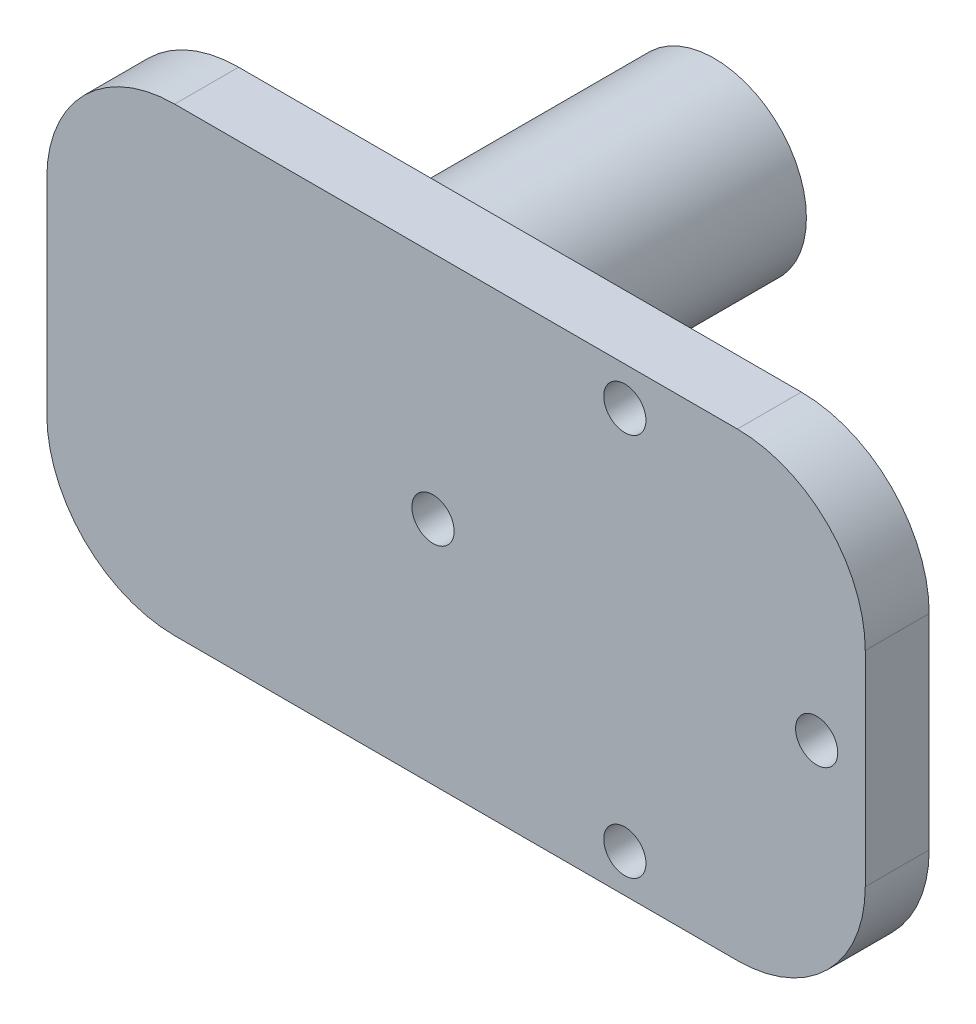
from build123d import *

# Parameters (mm, degrees)
SKETCH_1_R               = 7.2
SKETCH_1_R_2             = 4.2
EXTRUDE_1_DEPTH          = 7.5
EXTRUDE_START            = 20
SKETCH_2_R               = 7.2
EXTRUDE_2_DEPTH          = 20
SKETCH_3_R               = 17.2
SKETCH_3_R_2             = 7.2
EXTRUDE_3_DEPTH          = 3
SKETCH_4_R               = 1.65
CUT_EXTRUDE_1_DEPTH      = 3
PATTERN_CIRCULAR_1_COUNT = 4
SKETCH_5_W               = 64
SKETCH_5_H               = 36
EXTRUDE_4_DEPTH          = 5
SKETCH_6_R               = 1.65
CUT_EXTRUDE_2_DEPTH      = 50
FILLET_1_R               = 10
SKETCH_7_R               = 4.2
CUT_EXTRUDE_3_DEPTH      = 10


with BuildPart() as part:
    # 草图1 → 凸台-拉伸1 (new, symmetric)
    with BuildSketch(Plane.XY):
        Circle(SKETCH_1_R)
        Circle(SKETCH_1_R_2, mode=Mode.SUBTRACT)
    extrude(amount=EXTRUDE_1_DEPTH, both=True)

    # 草图2 → 凸台-拉伸2 (add)
    with BuildSketch(Plane.XY.offset(7.5).offset(EXTRUDE_START)):
        Circle(SKETCH_2_R)
    extrude(amount=-EXTRUDE_2_DEPTH)

    # 草图3 → 凸台-拉伸3 (add)
    with BuildSketch(Plane.XY.offset(27.5)):
        Circle(SKETCH_3_R)
        Circle(SKETCH_3_R_2, mode=Mode.SUBTRACT)
    extrude(amount=-EXTRUDE_3_DEPTH)

    # 草图4 → 切除-拉伸1 (cut)
    with BuildSketch(Plane(origin=(0, 0, 24.5), x_dir=(-1, 0, 0), z_dir=(0, 0, -1))):
        with Locations((0, 15)):
            Circle(SKETCH_4_R)
    cut_extrude_1 = extrude(amount=-CUT_EXTRUDE_1_DEPTH, mode=Mode.SUBTRACT)

    # 阵列(圆周)1: 切除-拉伸1 ×4 about axis
    pattern_circular_1_axis = Axis((0, 0, 0), (0, 0, 1))
    for i in range(1, PATTERN_CIRCULAR_1_COUNT):
        add(cut_extrude_1.rotate(pattern_circular_1_axis, i * 360 / PATTERN_CIRCULAR_1_COUNT), mode=Mode.SUBTRACT)

    # 草图5 → 凸台-拉伸4 (add)
    with BuildSketch(Plane.XY.offset(27.5)):
        with Locations((14.8, 0)):
            Rectangle(SKETCH_5_W, SKETCH_5_H)
    extrude(amount=-EXTRUDE_4_DEPTH)

    # 草图6 → 切除-拉伸2 (cut)
    with BuildSketch(Plane.XY.offset(27.5)):
        with Locations((28, 15)):
            Circle(SKETCH_6_R)
        with Locations((43, 0)):
            Circle(SKETCH_6_R)
        with Locations((28, -15)):
            Circle(SKETCH_6_R)
        with Locations((13, 0)):
            Circle(SKETCH_6_R)
    extrude(amount=-CUT_EXTRUDE_2_DEPTH, mode=Mode.SUBTRACT)

    # 圆角1
    fillet_1_edges = [part.edges().sort_by_distance(p)[0] for p in [
        (-17.2, -18, 25),
        (-17.2, 18, 25),
        (46.8, 18, 25),
        (46.8, -18, 25),
    ]]
    fillet(fillet_1_edges, radius=FILLET_1_R)

    # 草图7 → 切除-拉伸3 (cut)
    with BuildSketch(Plane(origin=(0, 0, 7.5), x_dir=(-1, 0, 0), z_dir=(0, 0, -1))):
        Circle(SKETCH_7_R)
    extrude(amount=-CUT_EXTRUDE_3_DEPTH, mode=Mode.SUBTRACT)


solid = part.part
